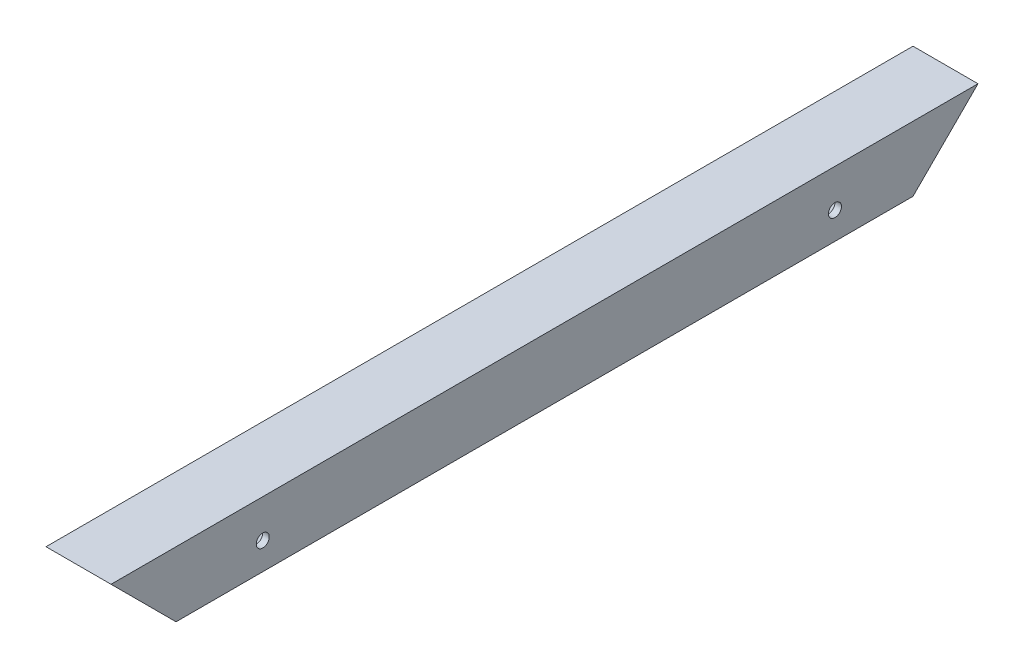
from build123d import *

# Parameters (mm, degrees)
SKETCH1_W               = 30
SKETCH1_H               = 30
BOSS_EXTRUDE1_DEPTH     = 400
SKETCH2_W               = 24
SKETCH2_H               = 24
CUT_EXTRUDE1_DEPTH      = 492
CUT_EXTRUDE3_DEPTH      = 402.958781438
CUT_EXTRUDE6_DEPTH      = 402.958781438
CUT_EXTRUDE7_DEPTH      = 402.958781438
CUT_EXTRUDE7_DEPTH_BACK = 402.958781438
SKETCH11_R              = 3


with BuildPart() as part:
    # Sketch1 → Boss-Extrude1 (new body)
    with BuildSketch(Plane.XY):
        with Locations((-30.141748722, 10.901003365)):
            Rectangle(SKETCH1_W, SKETCH1_H)
    extrude(amount=BOSS_EXTRUDE1_DEPTH)

    # Sketch2 → Cut-Extrude1 (cut)
    with BuildSketch(Plane.XY.offset(400)):
        with Locations((-30.141748722, 10.901003365)):
            Rectangle(SKETCH2_W, SKETCH2_H)
    extrude(amount=-CUT_EXTRUDE1_DEPTH, mode=Mode.SUBTRACT)

    # Sketch4 → Cut-Extrude3 (cut, through all)
    with BuildSketch(Plane(origin=(-15.141748722, 0, 0), x_dir=(0, 0, -1), z_dir=(1, 0, 0))):
        Polygon((0, 25.901003365), (-30, -4.098996635), (0, -4.098996635), align=None)
    extrude(amount=-CUT_EXTRUDE3_DEPTH, mode=Mode.SUBTRACT)

    # Sketch8 → Cut-Extrude6 (cut, through all)
    with BuildSketch(Plane(origin=(-15.141748722, 0, 0), x_dir=(0, 0, -1), z_dir=(1, 0, 0))):
        Polygon((-400, 25.901003365), (-370, -4.098996635), (-400, -4.098996635), align=None)
    extrude(amount=-CUT_EXTRUDE6_DEPTH, mode=Mode.SUBTRACT)

    # Sketch11 → Cut-Extrude7 (cut, two sides: drawn at the far end of the back side and taken through both)
    with BuildSketch(Plane(origin=(-15.141748722, 0, 0), x_dir=(0, 0, -1), z_dir=(1, 0, 0)).offset(-CUT_EXTRUDE7_DEPTH_BACK)):
        with Locations((-330, 8.401003365)):
            Circle(SKETCH11_R)
        with Locations((-66, 8.401003365)):
            Circle(SKETCH11_R)
    extrude(amount=CUT_EXTRUDE7_DEPTH + CUT_EXTRUDE7_DEPTH_BACK, mode=Mode.SUBTRACT)


solid = part.part
